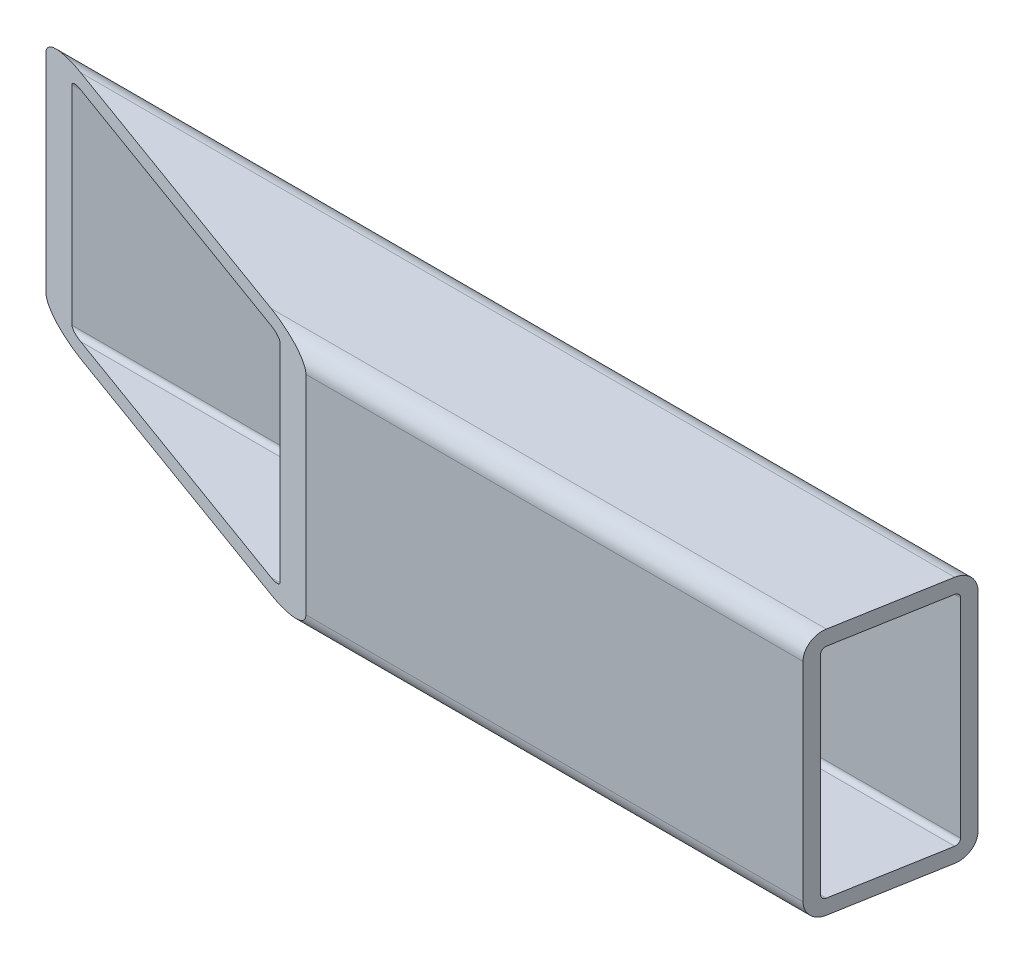
from build123d import *

# Parameters (mm, degrees)
SQUARE_TUBE_30_X_30_X_2_6_1_DEPTH = 200
CUT_EXTRUDE1_DEPTH                = 87
CUT_EXTRUDE2_DEPTH                = 137


with BuildPart() as part:
    # Sketch1 → Square tube 30 X 30 X 2.6(1) (new body)
    with BuildSketch(Plane.YZ):
        with BuildLine():
            Line((-21, -15), (21, -15))
            ThreePointArc((21, -15), (23.828427125, -13.828427125), (25, -11))
            Line((25, -11), (25, 11))
            ThreePointArc((25, 11), (23.828427125, 13.828427125), (21, 15))
            Line((21, 15), (-21, 15))
            ThreePointArc((-21, 15), (-23.828427125, 13.828427125), (-25, 11))
            Line((-25, 11), (-25, -11))
            ThreePointArc((-25, -11), (-23.828427125, -13.828427125), (-21, -15))
        make_face()
        with BuildLine():
            Line((-21, -12), (21, -12))
            ThreePointArc((21, -12), (21.707106781, -11.707106781), (22, -11))
            Line((22, -11), (22, 11))
            ThreePointArc((22, 11), (21.707106781, 11.707106781), (21, 12))
            Line((21, 12), (-21, 12))
            ThreePointArc((-21, 12), (-21.707106781, 11.707106781), (-22, 11))
            Line((-22, 11), (-22, -11))
            ThreePointArc((-22, -11), (-21.707106781, -11.707106781), (-21, -12))
        make_face(mode=Mode.SUBTRACT)
    extrude(amount=SQUARE_TUBE_30_X_30_X_2_6_1_DEPTH)

    # Sketch3 → Cut-Extrude1 (cut)
    with BuildSketch(Plane(origin=(0, 25, 0), x_dir=(1, 0, 0), z_dir=(0, 1, 0))):
        Polygon((188, 15), (182.710190579, -15), (200, -15), (200, 15), align=None)
    extrude(amount=-CUT_EXTRUDE1_DEPTH, mode=Mode.SUBTRACT)

    # Sketch4 → Cut-Extrude2 (cut)
    with BuildSketch(Plane(origin=(0, 25, 0), x_dir=(1, 0, 0), z_dir=(0, 1, 0))):
        Polygon((0, 15), (82.424322584, -15), (0, -15), align=None)
    extrude(amount=-CUT_EXTRUDE2_DEPTH, mode=Mode.SUBTRACT)


solid = part.part
